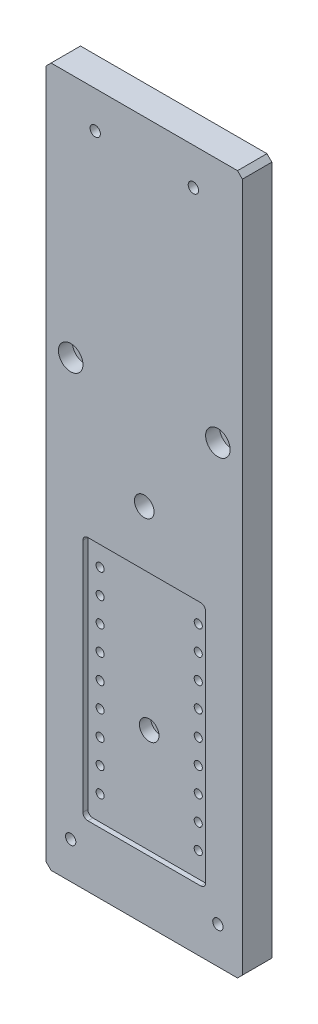
from build123d import *

# Parameters (mm, degrees)
SKETCH_1_W                = 80
SKETCH_1_H                = 285
EXTRUDE_1_DEPTH           = 12
HOLE_WIZARD_1_D           = 5.5
HOLE_WIZARD_1_CBORE_D     = 10
HOLE_WIZARD_1_CBORE_DEPTH = 5.7
HOLE_WIZARD_M5_1_D        = 4.2
CUT_EXTRUDE_2_DEPTH       = 2
HOLE_WIZARD_M4_1_D        = 3.3
HOLE_WIZARD_M5_2_D        = 4.2
CHAMFER_2_SIZE            = 2
HOLE_WIZARD_2_D           = 4.5
HOLE_WIZARD_2_CBORE_D     = 8
HOLE_WIZARD_2_CBORE_DEPTH = 6.6


with BuildPart() as part:
    # 草图1 → 凸台-拉伸1 (new body)
    with BuildSketch(Plane.XY):
        Rectangle(SKETCH_1_W, SKETCH_1_H)
    extrude(amount=EXTRUDE_1_DEPTH)

    # 打孔尺寸(%根据)内六角圆柱头螺钉的类型1 (through all)
    with Locations(Plane.XY.offset(12)):
        with Locations((30, 42.5), (-30, 42.5)):
            CounterBoreHole(HOLE_WIZARD_1_D / 2, HOLE_WIZARD_1_CBORE_D / 2, HOLE_WIZARD_1_CBORE_DEPTH)

    # M5 螺纹孔1 (through all)
    with Locations(Plane(origin=(0, 0, 0), x_dir=(-1, 0, 0), z_dir=(0, 0, -1))):
        with Locations((-20, 127.5), (20, 127.5)):
            Hole(HOLE_WIZARD_M5_1_D / 2)

    # 草图25 → 切除-拉伸2 (cut)
    with BuildSketch(Plane.XY.offset(12)):
        with BuildLine():
            Line((-23, -17.5), (23, -17.5))
            ThreePointArc((23, -17.5), (24.414213562, -18.085786438), (25, -19.5))
            Line((25, -19.5), (25, -115.5))
            ThreePointArc((25, -115.5), (24.414213562, -116.914213562), (23, -117.5))
            Line((23, -117.5), (-23, -117.5))
            ThreePointArc((-23, -117.5), (-24.414213562, -116.914213562), (-25, -115.5))
            Line((-25, -115.5), (-25, -19.5))
            ThreePointArc((-25, -19.5), (-24.414213562, -18.085786438), (-23, -17.5))
        make_face()
    extrude(amount=-CUT_EXTRUDE_2_DEPTH, mode=Mode.SUBTRACT)

    # M4 螺纹孔1 (through all)
    with Locations(Plane.XY.offset(10)):
        with Locations((-20, -27.5), (20, -27.5), (20, -37.5), (20, -47.5), (-20, -37.5), (-20, -47.5), (-20, -57.5), (20, -57.5), (-20, -67.5), (20, -67.5), (-20, -77.5), (20, -77.5), (-20, -87.5), (20, -87.5), (-20, -97.5), (20, -97.5), (-20, -107.5), (20, -107.5)):
            Hole(HOLE_WIZARD_M4_1_D / 2)

    # M5 螺纹孔2 (through all)
    with Locations(Plane.XY.offset(12)):
        with Locations((-30, -127.5), (30, -127.5)):
            Hole(HOLE_WIZARD_M5_2_D / 2)

    # 倒角2
    chamfer_2_edges = [part.edges().sort_by_distance(p)[0] for p in [
        (40, -142.5, 6),
        (-40, -142.5, 6),
        (-40, 142.5, 6),
        (40, 142.5, 6),
    ]]
    chamfer(chamfer_2_edges, length=CHAMFER_2_SIZE)

    # 打孔尺寸(%根据)内六角圆柱头螺钉的类型2 (through all)
    with Locations(Plane.XY.offset(12)):
        with Locations((0, 5), (0, -75)):
            CounterBoreHole(HOLE_WIZARD_2_D / 2, HOLE_WIZARD_2_CBORE_D / 2, HOLE_WIZARD_2_CBORE_DEPTH)


solid = part.part
